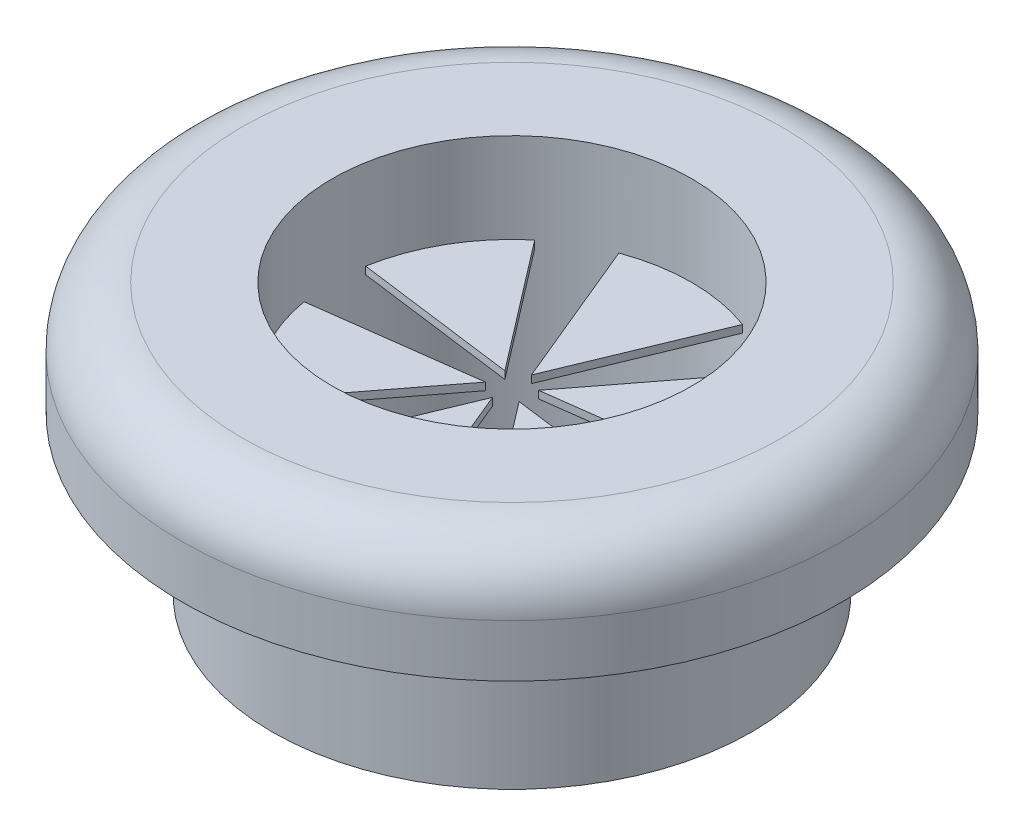
from build123d import *

# Parameters (mm, degrees)
SKETCH1_R           = 8
BOSS_EXTRUDE1_DEPTH = 5
SKETCH2_R           = 11
BOSS_EXTRUDE2_DEPTH = 4
CUT_EXTRUDE1_REACH  = 19.972
SKETCH3_R           = 6
BOSS_EXTRUDE3_START = -6
BOSS_EXTRUDE3_DEPTH = 0.25
SKETCH5_R           = 11
SKETCH5_R_2         = 10
CUT_EXTRUDE2_DEPTH  = 0.25
FILLET1_R           = 2


with BuildPart() as part:
    # Sketch1 → Boss-Extrude1 (new body)
    with BuildSketch(Plane(origin=(0, 0, 0), x_dir=(1, 0, 0), z_dir=(0, 1, 0))):
        with Locations(Location((0, 0, 0), (0, 0, 270))):
            Circle(SKETCH1_R)
    extrude(amount=BOSS_EXTRUDE1_DEPTH)

    # Sketch2 → Boss-Extrude2 (add)
    with BuildSketch(Plane(origin=(0, 5, 0), x_dir=(1, 0, 0), z_dir=(0, 1, 0))):
        with Locations(Location((0, 0, 0), (0, 0, 270))):
            Circle(SKETCH2_R)
    extrude(amount=BOSS_EXTRUDE2_DEPTH)

    # Sketch3 → Cut-Extrude1 (cut, up to next)
    with BuildSketch(Plane(origin=(0, 9, 0), x_dir=(1, 0, 0), z_dir=(0, 1, 0)), mode=Mode.PRIVATE) as cut_extrude1_sk1:
        with Locations(Location((0, 0, 0), (0, 0, 270))):
            Circle(SKETCH3_R)
    cut_extrude1_tool1 = extrude(cut_extrude1_sk1.sketch, amount=-CUT_EXTRUDE1_REACH, mode=Mode.PRIVATE) & part.part
    add(cut_extrude1_tool1.solids().sort_by_distance((0, 9, 0))[0], mode=Mode.SUBTRACT)

    # Sketch4 → Boss-Extrude3 (add)
    with BuildSketch(Plane.XZ.offset(BOSS_EXTRUDE3_START)):
        with BuildLine():
            Line((0, 0.65), (-2.064316872, 5.633701789))
            ThreePointArc((-2.064316872, 5.633701789), (0, 6), (2.064316872, 5.633701789))
            Line((2.064316872, 5.633701789), (0, 0.65))
        make_face()
        with BuildLine():
            Line((0.562916512, 0.325), (3.846770431, 4.604601747))
            ThreePointArc((3.846770431, 4.604601747), (5.196152423, 3), (5.911087303, 1.029100042))
            Line((5.911087303, 1.029100042), (0.562916512, 0.325))
        make_face()
        with BuildLine():
            Line((0.562916512, -0.325), (5.911087303, -1.029100042))
            ThreePointArc((5.911087303, -1.029100042), (5.196152423, -3), (3.846770431, -4.604601747))
            Line((3.846770431, -4.604601747), (0.562916512, -0.325))
        make_face()
        with BuildLine():
            Line((0, -0.65), (2.064316872, -5.633701789))
            ThreePointArc((2.064316872, -5.633701789), (0, -6), (-2.064316872, -5.633701789))
            Line((-2.064316872, -5.633701789), (0, -0.65))
        make_face()
        with BuildLine():
            Line((-0.562916512, -0.325), (-3.846770431, -4.604601747))
            ThreePointArc((-3.846770431, -4.604601747), (-5.196152423, -3), (-5.911087303, -1.029100042))
            Line((-5.911087303, -1.029100042), (-0.562916512, -0.325))
        make_face()
        with BuildLine():
            Line((-0.562916512, 0.325), (-5.911087303, 1.029100042))
            ThreePointArc((-5.911087303, 1.029100042), (-5.196152423, 3), (-3.846770431, 4.604601747))
            Line((-3.846770431, 4.604601747), (-0.562916512, 0.325))
        make_face()
    extrude(amount=BOSS_EXTRUDE3_DEPTH)

    # Sketch5 → Cut-Extrude2 (cut)
    with BuildSketch(Plane.XZ.offset(-5)):
        with Locations(Location((0, 0, 0), (0, 0, 270))):
            Circle(SKETCH5_R)
        with Locations(Location((0, 0, 0), (0, 0, 270))):
            Circle(SKETCH5_R_2, mode=Mode.SUBTRACT)
    extrude(amount=-CUT_EXTRUDE2_DEPTH, mode=Mode.SUBTRACT)

    # Fillet1
    fillet1_edges = [part.edges().sort_by_distance(p)[0] for p in [
        (0, 9, -11),
    ]]
    fillet(fillet1_edges, radius=FILLET1_R)


solid = part.part
